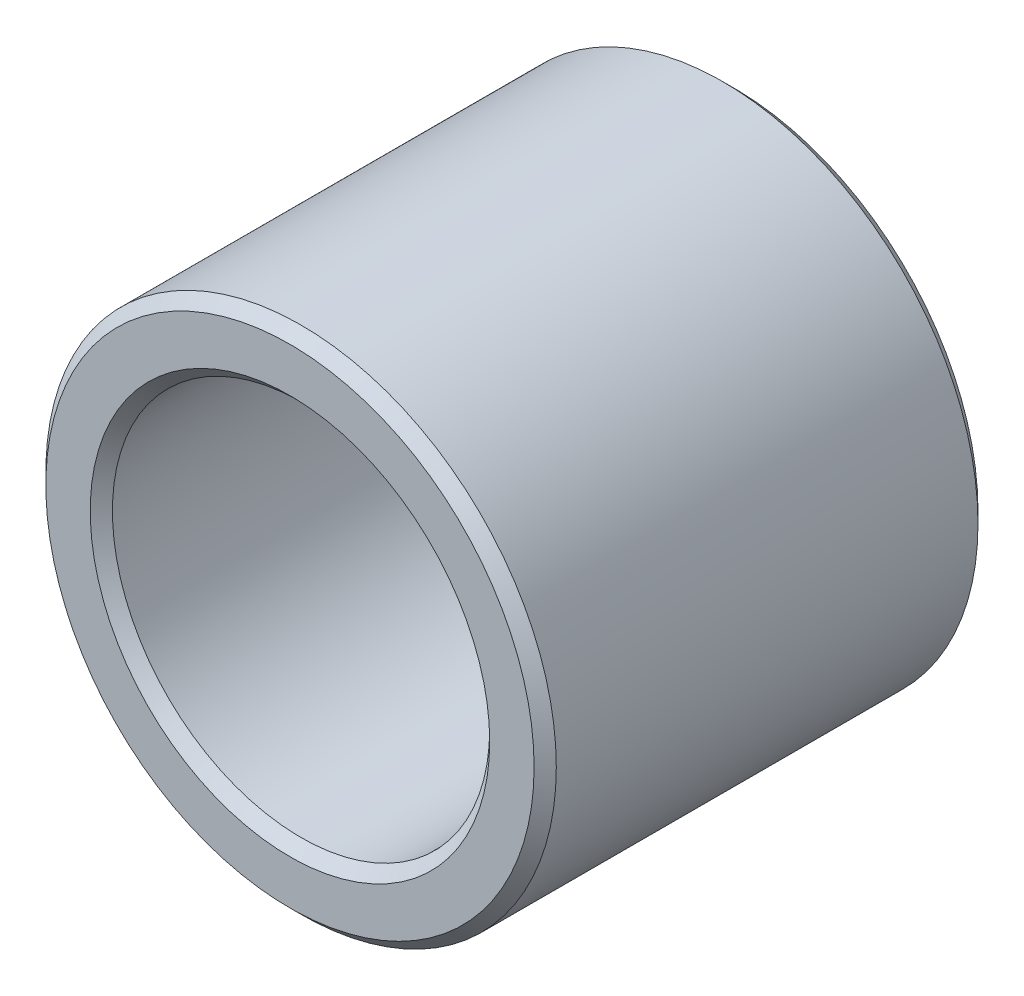
SolidWorks part; units mm, degrees
ref_plane "Front Plane" through (0, 0, 0) normal (0, 0, 1) x (1, 0, 0)
ref_plane "Top Plane" through (0, 0, 0) normal (0, 1, 0) x (1, 0, 0)
ref_plane "Right Plane" through (0, 0, 0) normal (1, 0, 0) x (0, 0, -1)
sketch "Sketch1" plane through (0, 0, 0) normal (0, 0, 1) x (1, 0, 0)
  circle A0 centre (0, 0) radius 11.5
  circle A1 centre (0, 0) radius 8.5
extrude "Boss-Extrude1" add sketch "Sketch1" along normal blind 20
chamfer "Chamfer1" distance 0.5 angle 45 4 edges at (11.5, 0, 0) (8.5, 0, 0) (11.5, 0, 20) (8.5, 0, 20)
